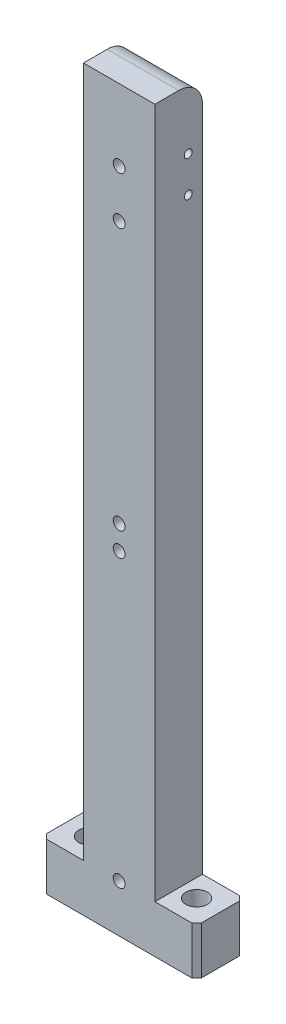
from build123d import *

# Parameters (mm, degrees)
EXTRUDE_1_DEPTH       = 20
HOLE_WIZARD_9_0_9_1_D = 9
HOLE_WIZARD_M6_1_D    = 5
FILLET_1_R            = 10
CHAMFER_1_SIZE        = 2
HOLE_WIZARD_M4_1_D    = 3.3


with BuildPart() as part:
    # 草图1 → 凸台-拉伸1 (new body)
    with BuildSketch(Plane.XY):
        Polygon((15, 310), (-15, 310), (-15, 20), (-32.5, 20), (-32.5, 0), (32.5, 0), (32.5, 20), (15, 20), align=None)
    extrude(amount=EXTRUDE_1_DEPTH)

    # Ø9.0 (9) 直径孔1 (through all)
    with Locations(Plane(origin=(0, 20, 0), x_dir=(1, 0, 0), z_dir=(0, 1, 0))):
        with Locations((22.5, -10), (-22.5, -10)):
            Hole(HOLE_WIZARD_9_0_9_1_D / 2)

    # M6 螺纹孔1 (through all)
    with Locations(Plane.XY.offset(20)):
        with Locations((0, 280), (0, 150), (0, 20), (0, 260), (0, 140)):
            Hole(HOLE_WIZARD_M6_1_D / 2)

    # 圆角1
    fillet_1_edges = [part.edges().sort_by_distance(p)[0] for p in [
        (0, 310, 0),
    ]]
    fillet(fillet_1_edges, radius=FILLET_1_R)

    # 倒角1
    chamfer_1_edges = [part.edges().sort_by_distance(p)[0] for p in [
        (-32.5, 10, 20),
        (32.5, 10, 20),
        (32.5, 10, 0),
        (-32.5, 10, 0),
    ]]
    chamfer(chamfer_1_edges, length=CHAMFER_1_SIZE)

    # M4 螺纹孔1 (through all)
    with Locations(Plane.ZY.offset(15)):
        with Locations((6, 285), (6, 270)):
            Hole(HOLE_WIZARD_M4_1_D / 2)


solid = part.part
